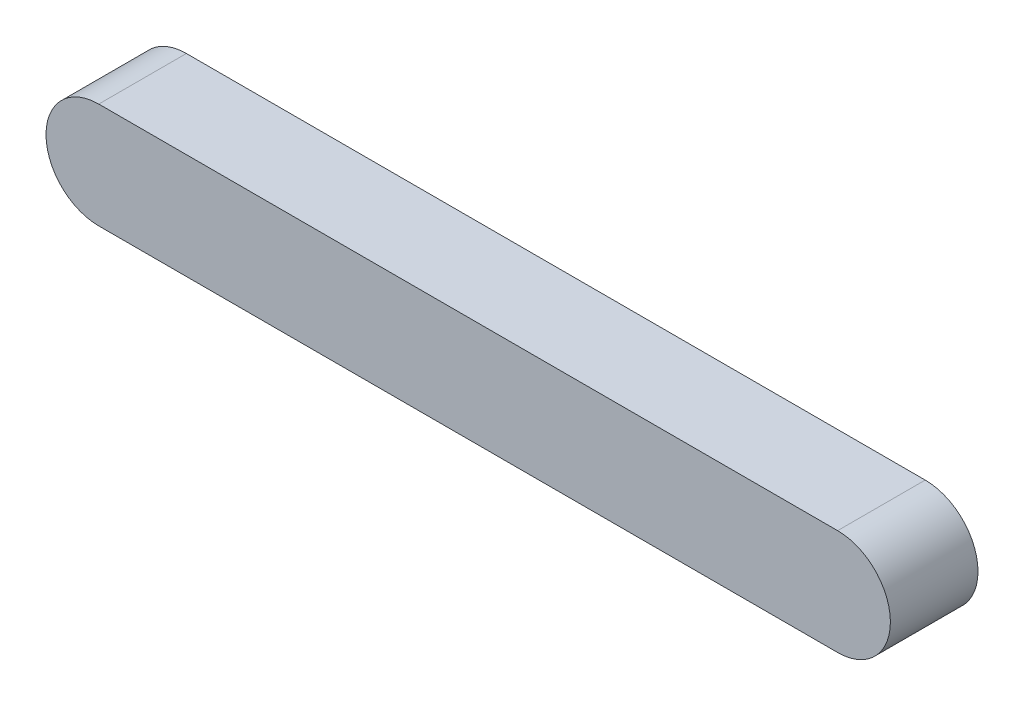
SolidWorks part; units mm, degrees
ref_plane "前视基准面" through (0, 0, 0) normal (0, 0, 1) x (1, 0, 0)
ref_plane "上视基准面" through (0, 0, 0) normal (0, 1, 0) x (1, 0, 0)
ref_plane "右视基准面" through (0, 0, 0) normal (1, 0, 0) x (0, 0, -1)
sketch "草图1" plane through (0, 0, 0) normal (0, 0, 1) x (1, 0, 0)
  line L0 (0, 0) -> (70, 0) construction
  line L1 (0, 5) -> (70, 5)
  line L2 (0, -5) -> (70, -5)
  arc A0 (0, 5) -> (0, -5) centre (0, 0) ccw
  arc A1 (70, -5) -> (70, 5) centre (70, 0) ccw
  point P3 (35, 0)
  dimension "D1" = 5
  dimension "D2" = 70
extrude "凸台-拉伸1" add sketch "草图1" along normal blind 8.3
